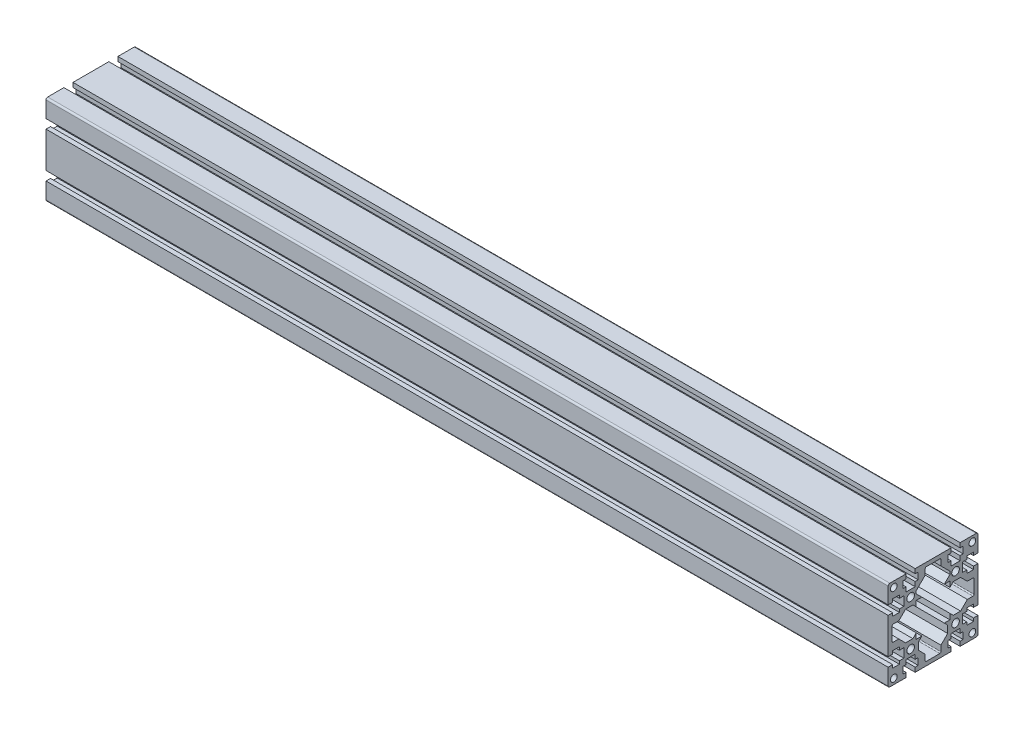
SolidWorks part; units mm, degrees
ref_plane "Front Plane" through (0, 0, 0) normal (0, 0, 1) x (1, 0, 0)
ref_plane "Top Plane" through (0, 0, 0) normal (0, 1, 0) x (1, 0, 0)
ref_plane "Right Plane" through (0, 0, 0) normal (1, 0, 0) x (0, 0, -1)
sketch "草图1" plane through (0, 0, 0) normal (0, 0, 1) x (1, 0, 0)
  line L0 (-530.3448, 0) -> (219.6552, 0)
  dimension "D1" = 750
other "Aluminium profile 80 X 80G X R1.5(1)"
ref_plane "Plane2" through (-530.3448, 0, 0) normal (1, 0, 0) x (0, 1, 0)
sketch "Sketch1" plane through (-530.3448, 0, 0) normal (1, 0, 0) x (0, 1, 0)
  line L0 (0, 40) -> (0, 0) construction
  line L1 (0, 0) -> (40, 0) construction
  line L2 (-24.05, 40) -> (-24.05, 36)
  line L3 (-38.5, 40) -> (-24.05, 40)
  line L4 (-40, 38.5) -> (-40, 24.05)
  line L5 (-38.5, -40) -> (-24.05, -40)
  line L6 (40, 38.5) -> (40, 24.05)
  line L7 (-24.05, 36) -> (-26.75, 36)
  line L8 (-26.75, 36) -> (-26.75, 30)
  line L9 (-26.75, 30) -> (-24.05, 30)
  line L10 (-24.05, 30) -> (-24.05, 26)
  line L11 (-24.05, 26) -> (-15.95, 26)
  line L12 (-15.95, 26) -> (-15.95, 30)
  line L13 (-15.95, 30) -> (-13.25, 30)
  line L14 (-13.25, 30) -> (-13.25, 36)
  line L15 (-13.25, 36) -> (-15.95, 36)
  line L16 (-15.95, 36) -> (-15.95, 40)
  line L17 (-40, 15.95) -> (-36, 15.95)
  line L18 (-36, 15.95) -> (-36, 13.25)
  line L19 (-15.95, 40) -> (15.95, 40)
  line L20 (-20, 20) -> (-20, 40) construction
  line L21 (20, 20) -> (20, 40) construction
  line L22 (15.95, 36) -> (15.95, 40)
  line L23 (13.25, 36) -> (15.95, 36)
  line L24 (13.25, 30) -> (13.25, 36)
  line L25 (15.95, 30) -> (13.25, 30)
  line L26 (-36, 13.25) -> (-30, 13.25)
  line L27 (-30, 13.25) -> (-30, 15.95)
  line L28 (-26, 15.95) -> (-26, 24.05)
  line L29 (-26, 24.05) -> (-30, 24.05)
  line L30 (-30, 24.05) -> (-30, 26.75)
  line L31 (-30, 26.75) -> (-36, 26.75)
  line L32 (-36, 26.75) -> (-36, 24.05)
  line L33 (-36, 24.05) -> (-40, 24.05)
  line L34 (-30, 15.95) -> (-26, 15.95)
  line L35 (15.95, 26) -> (15.95, 30)
  line L36 (24.05, 26) -> (15.95, 26)
  line L37 (24.05, 30) -> (24.05, 26)
  line L38 (26.75, 30) -> (24.05, 30)
  line L39 (26.75, 36) -> (26.75, 30)
  line L40 (24.05, 36) -> (26.75, 36)
  line L41 (24.05, 40) -> (24.05, 36)
  line L42 (24.05, -40) -> (24.05, -36)
  line L43 (24.05, -36) -> (26.75, -36)
  line L44 (26.75, -36) -> (26.75, -30)
  line L45 (26.75, -30) -> (24.05, -30)
  line L46 (24.05, -30) -> (24.05, -26)
  line L47 (24.05, -26) -> (15.95, -26)
  line L48 (15.95, -26) -> (15.95, -30)
  line L49 (15.95, -30) -> (13.25, -30)
  line L50 (13.25, -30) -> (13.25, -36)
  line L51 (13.25, -36) -> (15.95, -36)
  line L52 (15.95, -36) -> (15.95, -40)
  line L53 (-15.95, -36) -> (-15.95, -40)
  line L54 (-13.25, -36) -> (-15.95, -36)
  line L55 (-13.25, -30) -> (-13.25, -36)
  line L56 (-15.95, -30) -> (-13.25, -30)
  line L57 (-15.95, -26) -> (-15.95, -30)
  line L58 (-24.05, -26) -> (-15.95, -26)
  line L59 (-24.05, -30) -> (-24.05, -26)
  line L60 (-26.75, -30) -> (-24.05, -30)
  line L61 (-26.75, -36) -> (-26.75, -30)
  line L62 (-24.05, -36) -> (-26.75, -36)
  line L63 (-24.05, -40) -> (-24.05, -36)
  line L64 (-30, -15.95) -> (-26, -15.95)
  line L65 (-36, -26.75) -> (-36, -24.05)
  line L66 (-30, -26.75) -> (-36, -26.75)
  line L67 (-30, -24.05) -> (-30, -26.75)
  line L68 (-26, -24.05) -> (-30, -24.05)
  line L69 (-26, -15.95) -> (-26, -24.05)
  line L70 (-30, -13.25) -> (-30, -15.95)
  line L71 (-36, -13.25) -> (-30, -13.25)
  line L72 (-36, -15.95) -> (-36, -13.25)
  line L73 (36, 24.05) -> (40, 24.05)
  line L74 (40, 15.95) -> (36, 15.95)
  line L75 (36, -15.95) -> (36, -13.25)
  line L76 (36, -13.25) -> (30, -13.25)
  line L77 (30, -13.25) -> (30, -15.95)
  line L78 (26, -15.95) -> (26, -24.05)
  line L79 (26, -24.05) -> (30, -24.05)
  line L80 (30, -24.05) -> (30, -26.75)
  line L81 (30, -26.75) -> (36, -26.75)
  line L82 (36, -26.75) -> (36, -24.05)
  line L83 (30, -15.95) -> (26, -15.95)
  line L84 (30, 15.95) -> (26, 15.95)
  line L85 (36, 26.75) -> (36, 24.05)
  line L86 (30, 26.75) -> (36, 26.75)
  line L87 (30, 24.05) -> (30, 26.75)
  line L88 (26, 24.05) -> (30, 24.05)
  line L89 (26, 15.95) -> (26, 24.05)
  line L90 (30, 13.25) -> (30, 15.95)
  line L91 (36, 13.25) -> (30, 13.25)
  line L92 (36, 15.95) -> (36, 13.25)
  line L93 (-36, -15.95) -> (-40, -15.95)
  line L94 (-36, -24.05) -> (-40, -24.05)
  line L95 (36, -15.95) -> (40, -15.95)
  line L96 (36, -24.05) -> (40, -24.05)
  line L97 (-13, 18) -> (-10, 15)
  line L98 (-15, 15) -> (-10, 15)
  line L99 (-15, 15) -> (-15, 10)
  line L100 (-15, -15) -> (-10, -15)
  line L101 (15, 15) -> (15, 10)
  line L102 (-18, 13) -> (-15, 10)
  line L104 (13, 18) -> (10, 15)
  line L105 (13, -18) -> (10, -15)
  line L106 (20, -15) -> (15, -10)
  line L107 (-18, -13) -> (-15, -10)
  line L108 (-13, -18) -> (-10, -15)
  line L109 (15, -10) -> (15, -15)
  line L110 (10, 15) -> (15, 15)
  line L111 (-15, -10) -> (-15, -15)
  line L112 (10, -15) -> (15, -15)
  line L113 (15, 10) -> (20, 15)
  line L235 (24.05, 40) -> (38.5, 40)
  line L249 (-40, 15.95) -> (-40, -15.95)
  line L250 (-20, 20) -> (-26, 20) construction
  line L264 (40, 15.95) -> (40, -15.95)
  line L265 (-13, 24.5) -> (-7, 30.5)
  line L266 (-7, 30.5) -> (-7, 35.5)
  line L267 (7, 35.5) -> (7, 30.5)
  line L268 (7, 30.5) -> (13, 24.5)
  line L269 (-6, -36.5) -> (6, -36.5)
  line L270 (-13, 24.5) -> (-13, 18)
  line L271 (-35.5, 7) -> (-30.5, 7)
  line L272 (-30.5, 7) -> (-24.5, 13)
  line L273 (-24.5, 13) -> (-18, 13)
  line L274 (13, 24.5) -> (13, 18)
  line L275 (-15.95, -40) -> (15.95, -40)
  line L276 (35.5, 7) -> (30.5, 7)
  line L277 (30.5, 7) -> (22.5, 15)
  line L278 (24.05, -40) -> (38.5, -40)
  line L279 (20, 15) -> (22.5, 15)
  line L333 (-13, -24.5) -> (-13, -18)
  line L336 (-13, -24.5) -> (-7, -30.5)
  line L385 (-7, -30.5) -> (-7, -35.5)
  line L386 (-36.5, 6) -> (-36.5, -6)
  line L387 (7, -35.5) -> (7, -30.5)
  line L429 (7, -30.5) -> (13, -24.5)
  line L430 (13, -24.5) -> (13, -18)
  line L494 (20, -15) -> (22.5, -15)
  line L496 (30.5, -7) -> (22.5, -15)
  line L497 (35.5, -7) -> (30.5, -7)
  line L498 (-24.5, -13) -> (-18, -13)
  line L499 (-30.5, -7) -> (-24.5, -13)
  line L500 (-35.5, -7) -> (-30.5, -7)
  line L512 (40, -24.05) -> (40, -38.5)
  line L519 (-40, -24.05) -> (-40, -38.5)
  line L520 (-6, 36.5) -> (6, 36.5)
  line L523 (36.5, 6) -> (36.5, -6)
  circle A0 centre (-20, 20) radius 3.4
  circle A2 centre (20, 20) radius 3.4
  circle A3 centre (20, -20) radius 3.4
  circle A7 centre (-20, -20) radius 3.4
  arc A8 (-38.5, 40) -> (-40, 38.5) centre (-38.5, 38.5) ccw
  arc A9 (-40, -38.5) -> (-38.5, -40) centre (-38.5, -38.5) ccw
  arc A10 (38.5, -40) -> (40, -38.5) centre (38.5, -38.5) ccw
  arc A11 (38.5, 40) -> (40, 38.5) centre (38.5, 38.5) cw
  circle A12 centre (-35, 35) radius 3
  circle A13 centre (35, 35) radius 3
  circle A14 centre (35, -35) radius 3
  arc A15 (-6, 36.5) -> (-7, 35.5) centre (-6, 35.5) ccw
  arc A16 (6, 36.5) -> (7, 35.5) centre (6, 35.5) cw
  arc A17 (-36.5, 6) -> (-35.5, 7) centre (-35.5, 6) cw
  arc A18 (-36.5, -6) -> (-35.5, -7) centre (-35.5, -6) ccw
  arc A19 (36.5, -6) -> (35.5, -7) centre (35.5, -6) cw
  arc A20 (36.5, 6) -> (35.5, 7) centre (35.5, 6) ccw
  arc A21 (6, -36.5) -> (7, -35.5) centre (6, -35.5) ccw
  arc A22 (-6, -36.5) -> (-7, -35.5) centre (-6, -35.5) cw
  point P48 (-20, 20)
  point P97 (0, 0)
  point P104 (-7, 36.5)
  point P185 (40, 40)
  point P187 (40, -40)
  point P188 (-40, -40)
  point P190 (-40, 40)
  dimension "D1" = 80
  dimension "D2" = 80
  dimension "D3" = 20
  dimension "D4" = 8.1
  dimension "D5" = 45
  dimension "D6" = 7
  dimension "D7" = 13.5
  dimension "D8" = 6
  dimension "D12" = 5
  dimension "D13" = 5
  dimension "D14" = 20
  dimension "D18" = 1
  dimension "D19" = 14
  dimension "D15" = 6.8
  dimension "D27" = 45
  dimension "D20" = 1.5
  dimension "D11" = 6
  dimension "D9" = 4
  dimension "D10" = 14
  dimension "D16" = 14
  dimension "D17" = 45
  dimension "D21" = 3.5
  dimension "D22" = 3.5
  dimension "D23" = 73
  dimension "D24" = 30
  dimension "D25" = 30
  dimension "D26" = 45
  dimension "D28" = 5
sketch "Sketch10" plane through (219.6552, 0, 0) normal (1, 0, 0) x (0, 0, -1)
  circle A0 centre (35, -35) radius 3
  circle A1 centre (-35, -35) radius 3 construction
  circle A2 centre (35, 35) radius 3 construction
  dimension "D1" = 6
  dimension "D2" = 70
  dimension "D3" = 70
extrude "Cut-Extrude1" cut sketch "Sketch10" against normal through all
